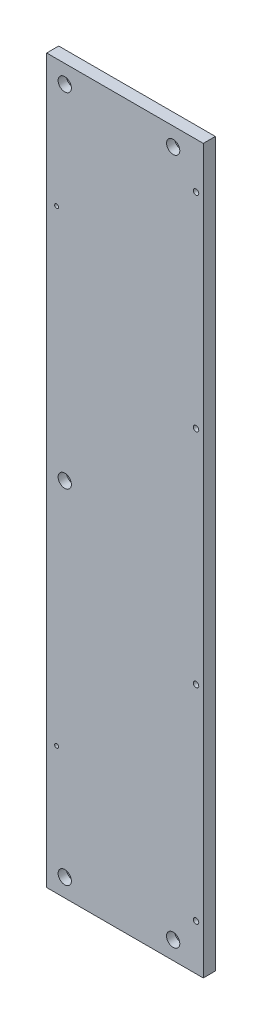
SolidWorks part; units mm, degrees
ref_plane "前视基准面" through (0, 0, 0) normal (0, 0, 1) x (1, 0, 0)
ref_plane "上视基准面" through (0, 0, 0) normal (0, 1, 0) x (1, 0, 0)
ref_plane "右视基准面" through (0, 0, 0) normal (1, 0, 0) x (0, 0, -1)
sketch "草图1" plane through (0, 0, 0) normal (0, 0, 1) x (1, 0, 0)
  line L1 (-65, 300) -> (65, 300)
  line L2 (-65, 300) -> (-65, -300)
  line L3 (-65, -300) -> (65, -300)
  line L4 (65, 300) -> (65, -300)
  line L5 (-65, 300) -> (65, -300) construction
  line L6 (-65, -300) -> (65, 300) construction
  point P0 (0, 0)
  dimension "D1" = 600
  dimension "D2" = 130
extrude "凸台-拉伸1" add sketch "草图1" along normal blind 10
hole_wizard "打孔尺寸根据内六角圆柱头螺钉的类型2" positions "草图3" profile "草图2" counterbore size "M6" standard "Gb" end condition through all
sketch "草图3" plane through (0, 0, 10) normal (0, 0, 1) x (1, 0, 0)
  line L0 (40, 285) -> (-50, 285) construction
  line L1 (-50, 285) -> (-50, 0) construction
  line L2 (-50, 0) -> (-50, -285) construction
  line L5 (40, 285) -> (40, -285) construction
  line L6 (40, -285) -> (-50, -285) construction
  line L8 (-65, 300) -> (-65, -300) construction
  line L9 (65, 300) -> (-65, 300) construction
  line L10 (-65, -300) -> (65, -300) construction
  line L11 (14.149, 0) -> (-62.0766, 0) construction
  point P0 (-50, 285)
  point P2 (-50, 0)
  point P4 (-50, -285)
  point P6 (40, 285)
  point P8 (40, -285)
  dimension "D1" = 15
  dimension "D2" = 15
  dimension "D3" = 15
  dimension "D4" = 90
sketch "草图2" plane through (-50, 285, 10) normal (1, 0, 0) x (0, -1, 0)
  line L0 (0, 0) -> (0, 10)
  line L1 (0, 10) -> (3.3, 10)
  line L3 (3.3, 10) -> (3.3, 6.8)
  line L4 (3.3, 6.8) -> (5.5, 6.8)
  line L5 (5.5, 6.8) -> (5.5, 0)
  line L7 (5.5, 0) -> (0, 0)
  line L11 (0, -6.35) -> (0, 107.95) construction
  dimension "通孔孔直径" = 6.6
  dimension "通孔孔深度" = 10
  dimension "柱形沉头孔直径" = 11
  dimension "柱形沉头孔深度" = 6.8
hole_wizard "M4 螺纹孔2" positions "草图7" profile "草图6" tap size "M4" standard "Iso" end condition through all
sketch "草图7" plane through (0, 0, 10) normal (0, 0, 1) x (1, 0, 0)
  point P0 (-56.75, 194)
  point P2 (-56.75, -194)
sketch "草图6" plane through (-56.75, 194, 10) normal (1, 0, 0) x (0, -1, 0)
  line L0 (0, 0) -> (0, 10)
  line L1 (0, 10) -> (1.65, 10)
  line L2 (1.65, 10) -> (1.65, 0)
  line L5 (1.65, 0) -> (0, 0)
  line L11 (0, -6.35) -> (0, 107.95) construction
  dimension "通孔螺纹孔钻头直径" = 3.3
  dimension "通孔螺纹孔钻头深度" = 10
cosmetic thread "孔螺蚊线3"
cosmetic thread "孔螺蚊线4"
hole_wizard "打孔尺寸根据内六角圆柱头螺钉的类型2" positions "草图9" profile "草图8" counterbore size "M4" standard "Gb" end condition through all
sketch "草图9" plane through (0, 0, 0) normal (0, 0, -1) x (-1, 0, 0)
  line L0 (-65, -300) -> (-65, 300) construction
  line L1 (-65, 300) -> (65, 300) construction
  line L2 (65, -300) -> (-65, -300) construction
  point P0 (-59, -262)
  point P2 (-59, -92)
  point P4 (-59, 92)
  point P6 (-59, 262)
  dimension "D1" = 6
  dimension "D2" = 38
  dimension "D3" = 170
  dimension "D4" = 38
  dimension "D5" = 170
sketch "草图8" plane through (59, -262, 0) normal (1, 0, 0) x (0, 1, 0)
  line L0 (0, 0) -> (0, 10)
  line L1 (0, 10) -> (2.25, 10)
  line L3 (2.25, 10) -> (2.25, 4.6)
  line L4 (2.25, 4.6) -> (4, 4.6)
  line L5 (4, 4.6) -> (4, 0)
  line L7 (4, 0) -> (0, 0)
  line L11 (0, -6.35) -> (0, 107.95) construction
  dimension "通孔孔直径" = 4.5
  dimension "通孔孔深度" = 10
  dimension "柱形沉头孔直径" = 8
  dimension "柱形沉头孔深度" = 4.6
